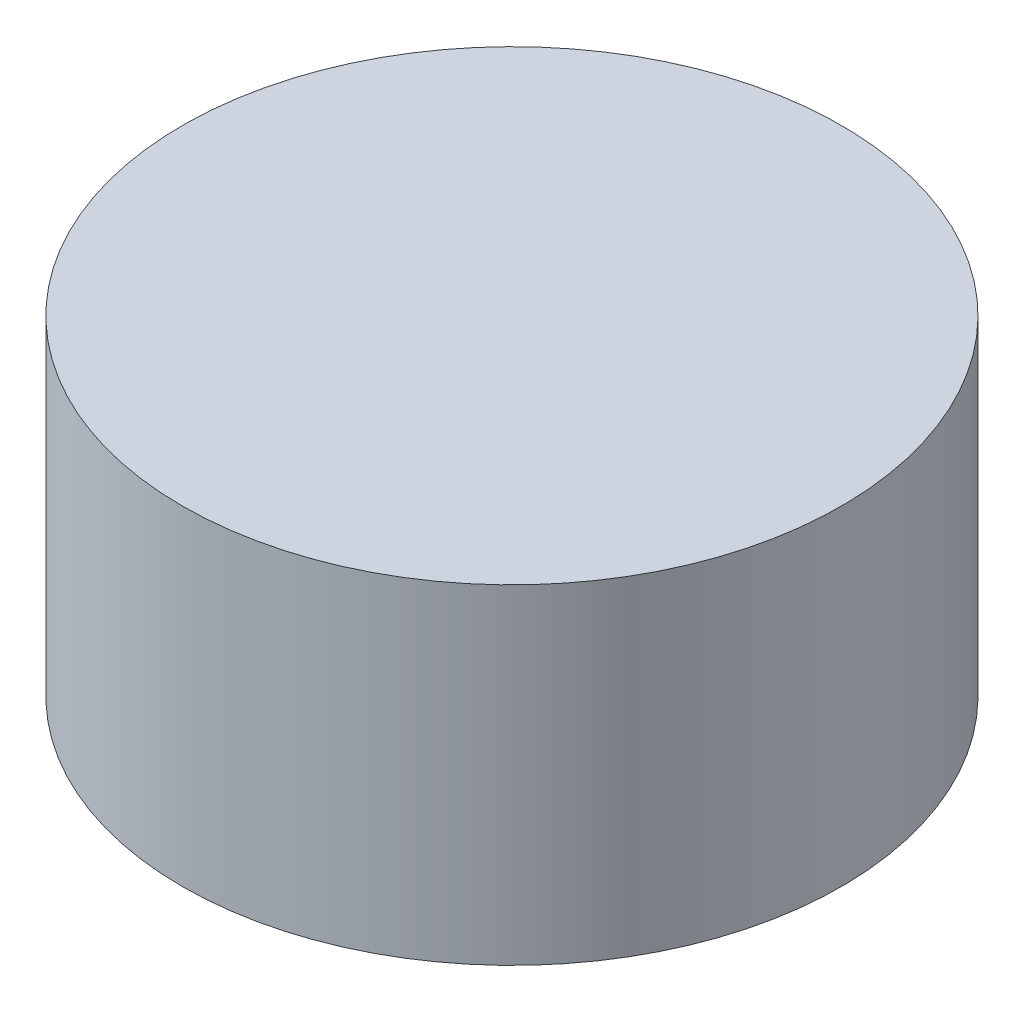
SolidWorks part; units mm, degrees
ref_plane "Front Plane" through (0, 0, 0) normal (0, 0, 1) x (1, 0, 0)
ref_plane "Top Plane" through (0, 0, 0) normal (0, 1, 0) x (1, 0, 0)
ref_plane "Right Plane" through (0, 0, 0) normal (1, 0, 0) x (0, 0, -1)
sketch "Sketch1" plane through (0, 0, 0) normal (0, 1, 0) x (1, 0, 0)
  circle A0 centre (0, 0) radius 5
extrude "Boss-Extrude1" add sketch "Sketch1" along normal blind 5
